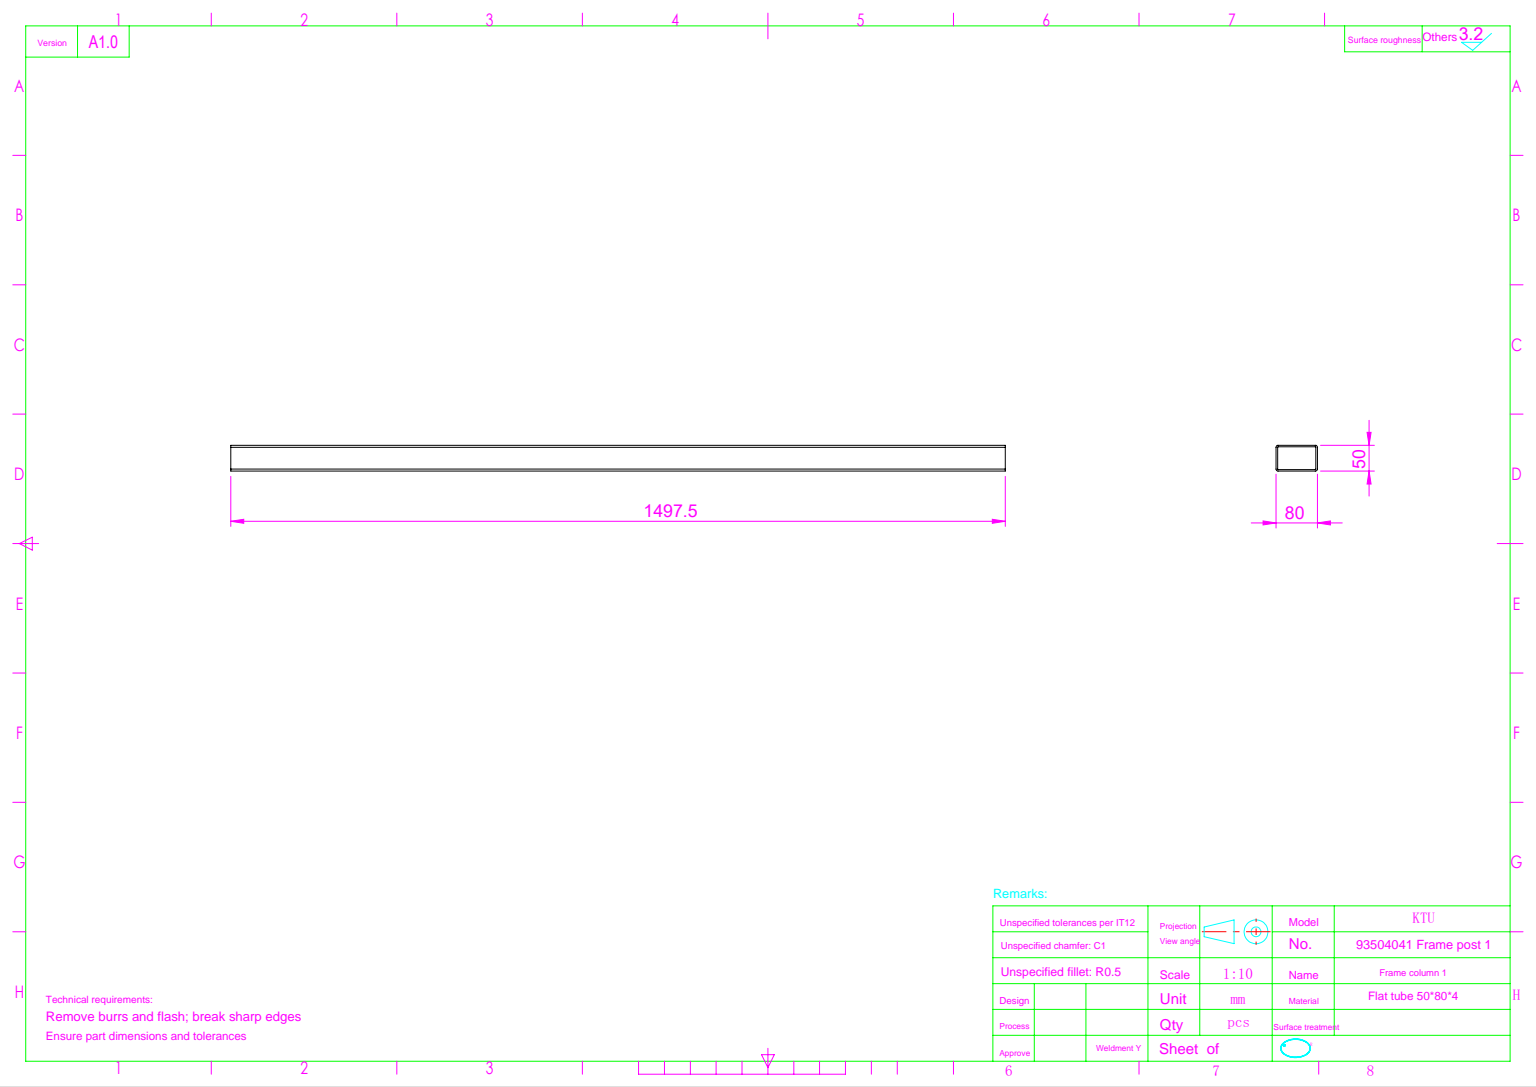
from build123d import *

# Parameters (mm, degrees)
EXTRUDE_1_DEPTH = 748.75


with BuildPart() as part:
    # 草图1 → 拉伸-薄壁1 (new, symmetric)
    with BuildSketch(Plane.XY):
        with BuildLine():
            Line((-36, 25), (36, 25))
            ThreePointArc((36, 25), (38.828427125, 23.828427125), (40, 21))
            Line((40, 21), (40, -21))
            ThreePointArc((40, -21), (38.828427125, -23.828427125), (36, -25))
            Line((36, -25), (-36, -25))
            ThreePointArc((-36, -25), (-38.828427125, -23.828427125), (-40, -21))
            Line((-40, -21), (-40, 21))
            ThreePointArc((-40, 21), (-38.828427125, 23.828427125), (-36, 25))
        make_face()
        with BuildLine():
            Line((-36, 22), (36, 22))
            ThreePointArc((36, 22), (36.707106781, 21.707106781), (37, 21))
            Line((37, 21), (37, -21))
            ThreePointArc((37, -21), (36.707106781, -21.707106781), (36, -22))
            Line((36, -22), (-36, -22))
            ThreePointArc((-36, -22), (-36.707106781, -21.707106781), (-37, -21))
            Line((-37, -21), (-37, 21))
            ThreePointArc((-37, 21), (-36.707106781, 21.707106781), (-36, 22))
        make_face(mode=Mode.SUBTRACT)
    extrude(amount=EXTRUDE_1_DEPTH, both=True)


solid = part.part
